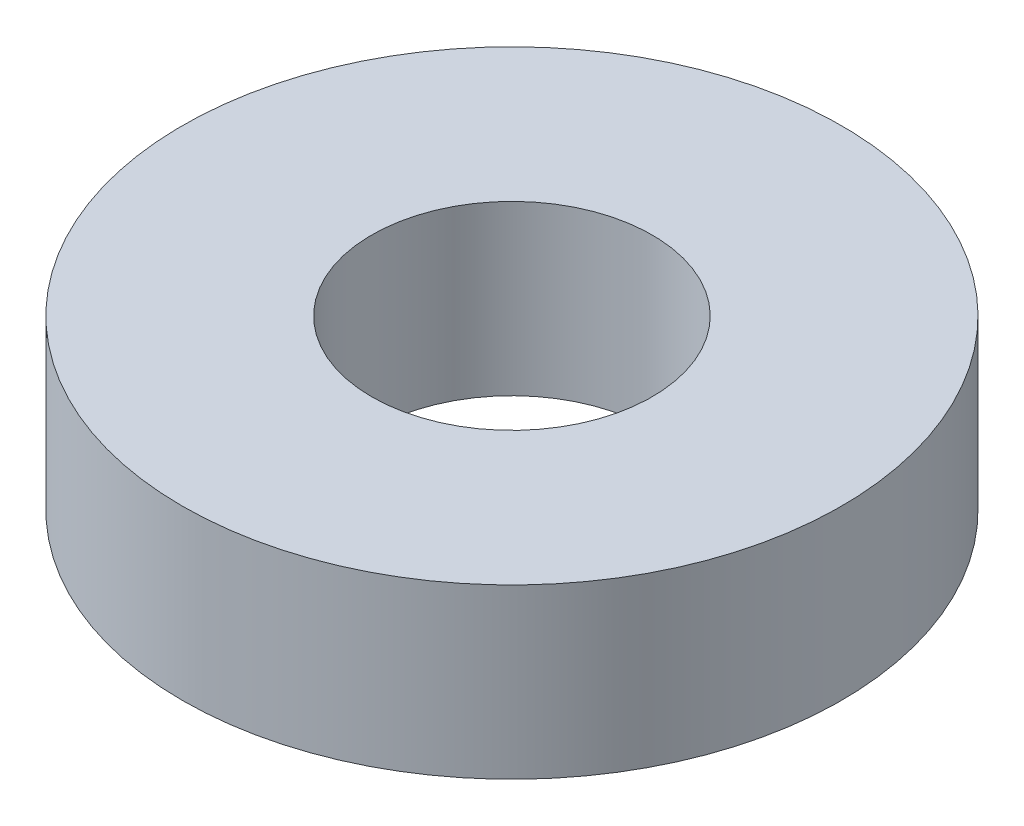
SolidWorks part; units mm, degrees
ref_plane "Front Plane" through (0, 0, 0) normal (0, 0, 1) x (1, 0, 0)
ref_plane "Top Plane" through (0, 0, 0) normal (0, 1, 0) x (1, 0, 0)
ref_plane "Right Plane" through (0, 0, 0) normal (1, 0, 0) x (0, 0, -1)
sketch "Sketch1" plane through (0, 0, 0) normal (0, 1, 0) x (1, 0, 0)
  circle A0 centre (0, 0) radius 23.5
  circle A1 centre (0, 0) radius 10
  dimension "D1" = 47
  dimension "D2" = 20
extrude "Boss-Extrude1" add sketch "Sketch1" along normal blind 12
